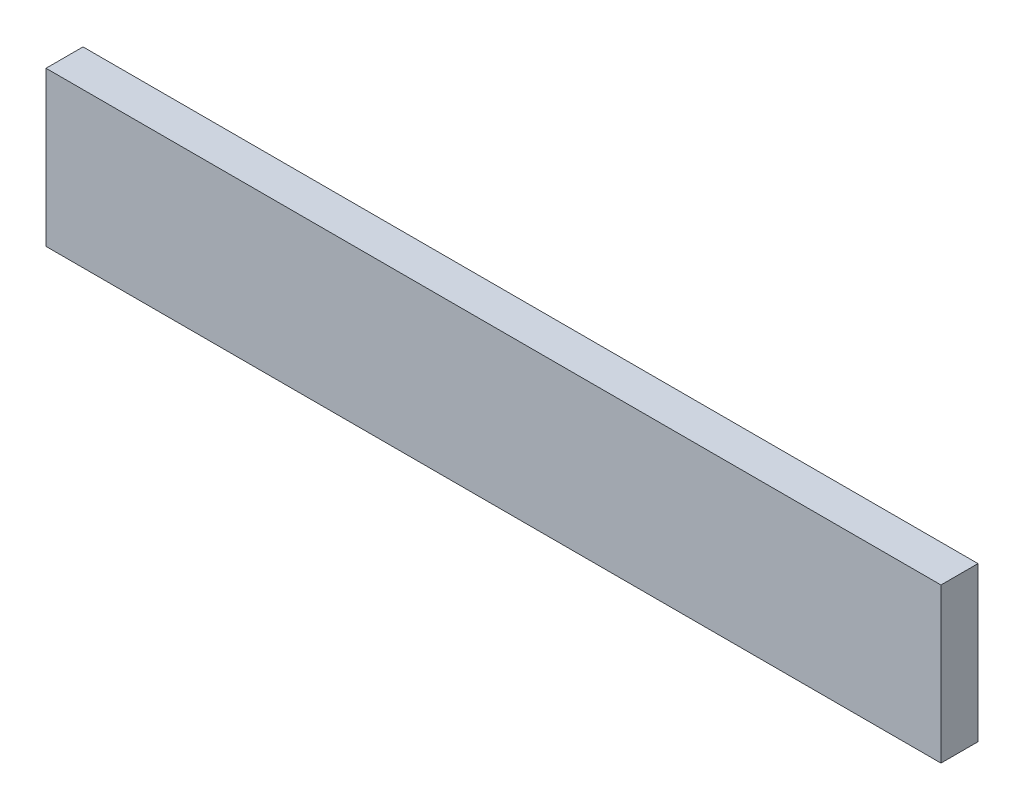
from build123d import *

# Parameters (mm, degrees)
SKETCH1_W           = 290
SKETCH1_H           = 50
BOSS_EXTRUDE1_DEPTH = 12


with BuildPart() as part:
    # Sketch1 → Boss-Extrude1 (new body)
    with BuildSketch(Plane.XY):
        with Locations((145, 25)):
            Rectangle(SKETCH1_W, SKETCH1_H)
    extrude(amount=BOSS_EXTRUDE1_DEPTH)


solid = part.part
